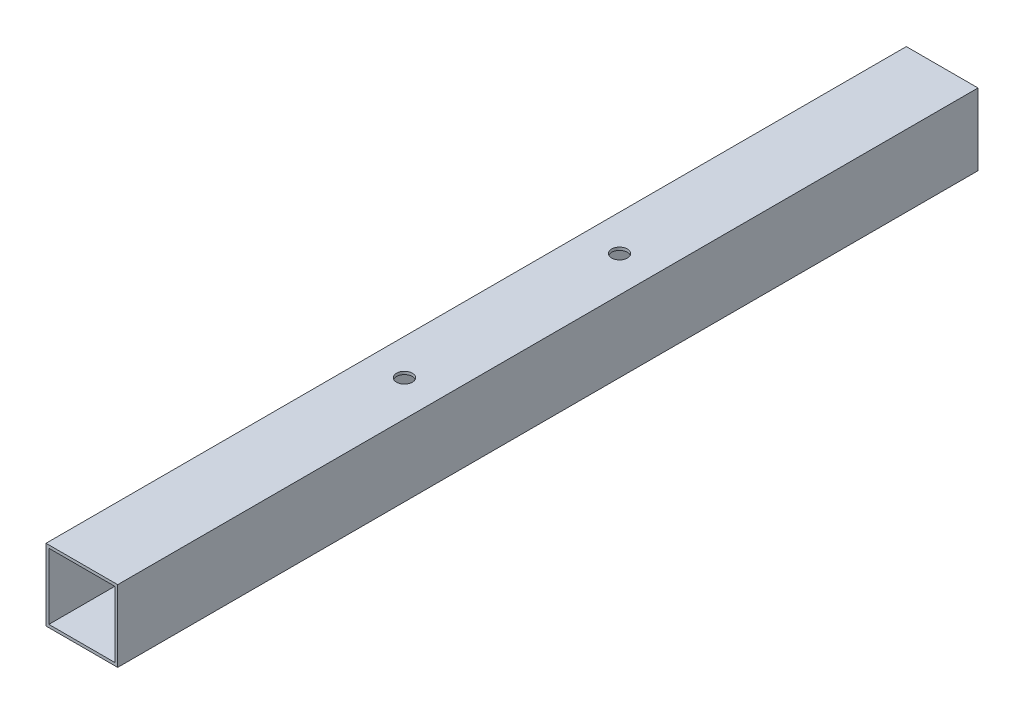
SolidWorks part; units mm, degrees
material "AISI 304"
ref_plane "Front Plane" through (0, 0, 0) normal (0, 0, 1) x (1, 0, 0)
ref_plane "Top Plane" through (0, 0, 0) normal (0, 1, 0) x (1, 0, 0)
ref_plane "Right Plane" through (0, 0, 0) normal (1, 0, 0) x (0, 0, -1)
sketch "Sketch1" plane through (0, 0, 0) normal (0, 0, 1) x (1, 0, 0)
  line L1 (-25, -25) -> (25, -25)
  line L2 (-25, -25) -> (-25, 25)
  line L3 (-25, 25) -> (25, 25)
  line L4 (25, -25) -> (25, 25)
  line L5 (-25, -25) -> (25, 25) construction
  line L6 (-25, 25) -> (25, -25) construction
  line L7 (-23, -23) -> (23, -23)
  line L8 (-23, -23) -> (-23, 23)
  line L9 (-23, 23) -> (23, 23)
  line L10 (23, -23) -> (23, 23)
  line L11 (-23, -23) -> (23, 23) construction
  line L12 (-23, 23) -> (23, -23) construction
  point P0 (0, 0)
  point P6 (0, 0)
  dimension "D1" = 50
  dimension "D2" = 50
  dimension "D3" = 46
  dimension "D4" = 46
extrude "Boss-Extrude1" add sketch "Sketch1" along normal blind 600
sketch "Sketch2" plane through (0, 25, 0) normal (0, 1, 0) x (1, 0, 0)
  circle A0 centre (0, -225) radius 5.5
  circle A1 centre (0, -375) radius 5.5
extrude "Cut-Extrude1" cut sketch "Sketch2" against normal blind 50
